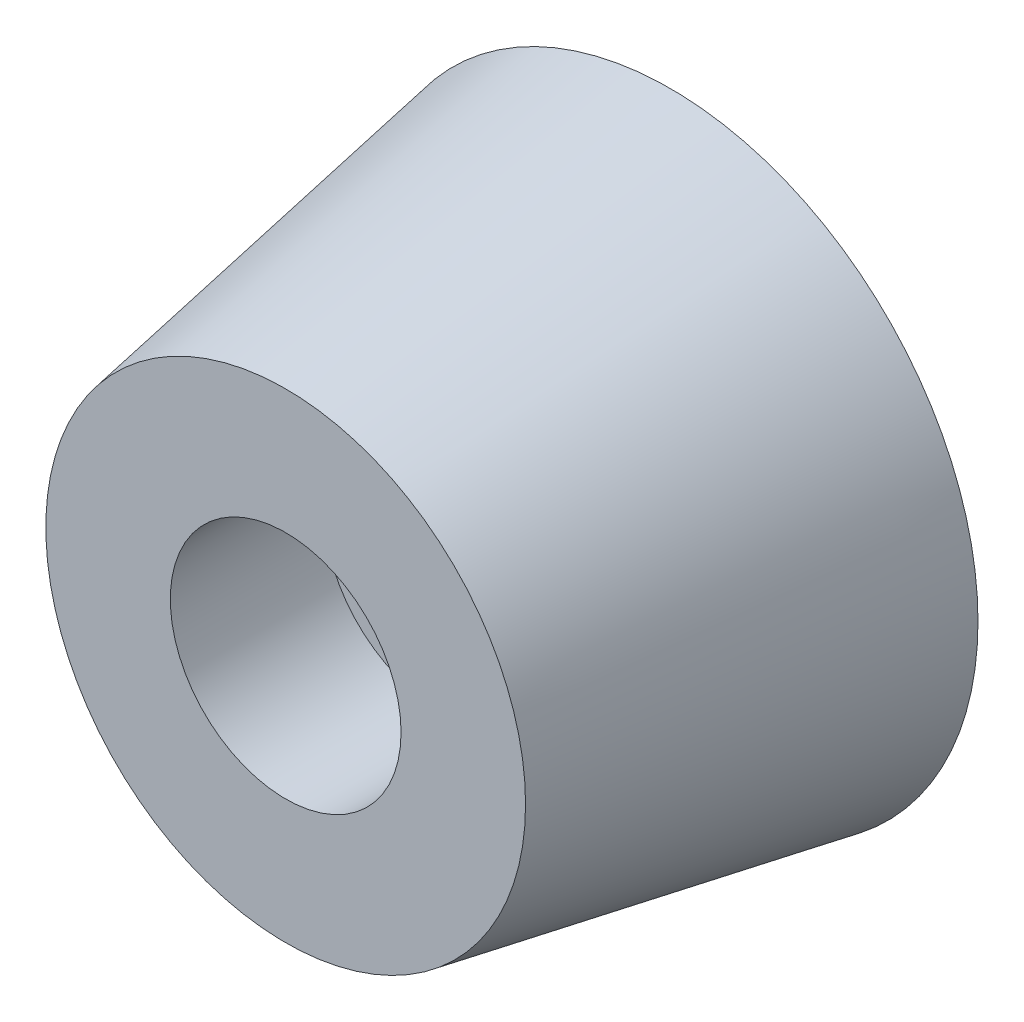
SolidWorks part; units mm, degrees
ref_plane "前视基准面" through (0, 0, 0) normal (0, 0, 1) x (1, 0, 0)
ref_plane "上视基准面" through (0, 0, 0) normal (0, 1, 0) x (1, 0, 0)
ref_plane "右视基准面" through (0, 0, 0) normal (1, 0, 0) x (0, 0, -1)
sketch "草图1" plane through (0, 0, 0) normal (0, 0, 1) x (1, 0, 0)
  circle A0 centre (0, 0) radius 8
  dimension "D1" = 16
extrude "凸台-拉伸1" add sketch "草图1" along normal blind 10 draft 10
hole_wizard "打孔尺寸(%根据)内六角圆柱头螺钉的类型1" positions "草图2" profile "草图4" counterbore size "M3" standard "GB" end condition through all
sketch "草图2" plane through (0, 0, 10) normal (0, 0, 1) x (1, 0, 0)
  point P0 (0, 0)
sketch "草图4" plane through (0, 0, 10) normal (1, 0, 0) x (0, -1, 0)
  line L0 (0, 0) -> (0, 10)
  line L1 (0, 10) -> (1.7, 10)
  line L3 (1.7, 10) -> (1.7, 4)
  line L4 (1.7, 4) -> (3, 4)
  line L5 (3, 4) -> (3, 0)
  line L7 (3, 0) -> (0, 0)
  line L11 (0, -6.35) -> (0, 107.95) construction
  dimension "通孔孔直径" = 3.4
  dimension "通孔孔深度" = 10
  dimension "柱形沉头孔直径" = 6
  dimension "柱形沉头孔深度" = 4
